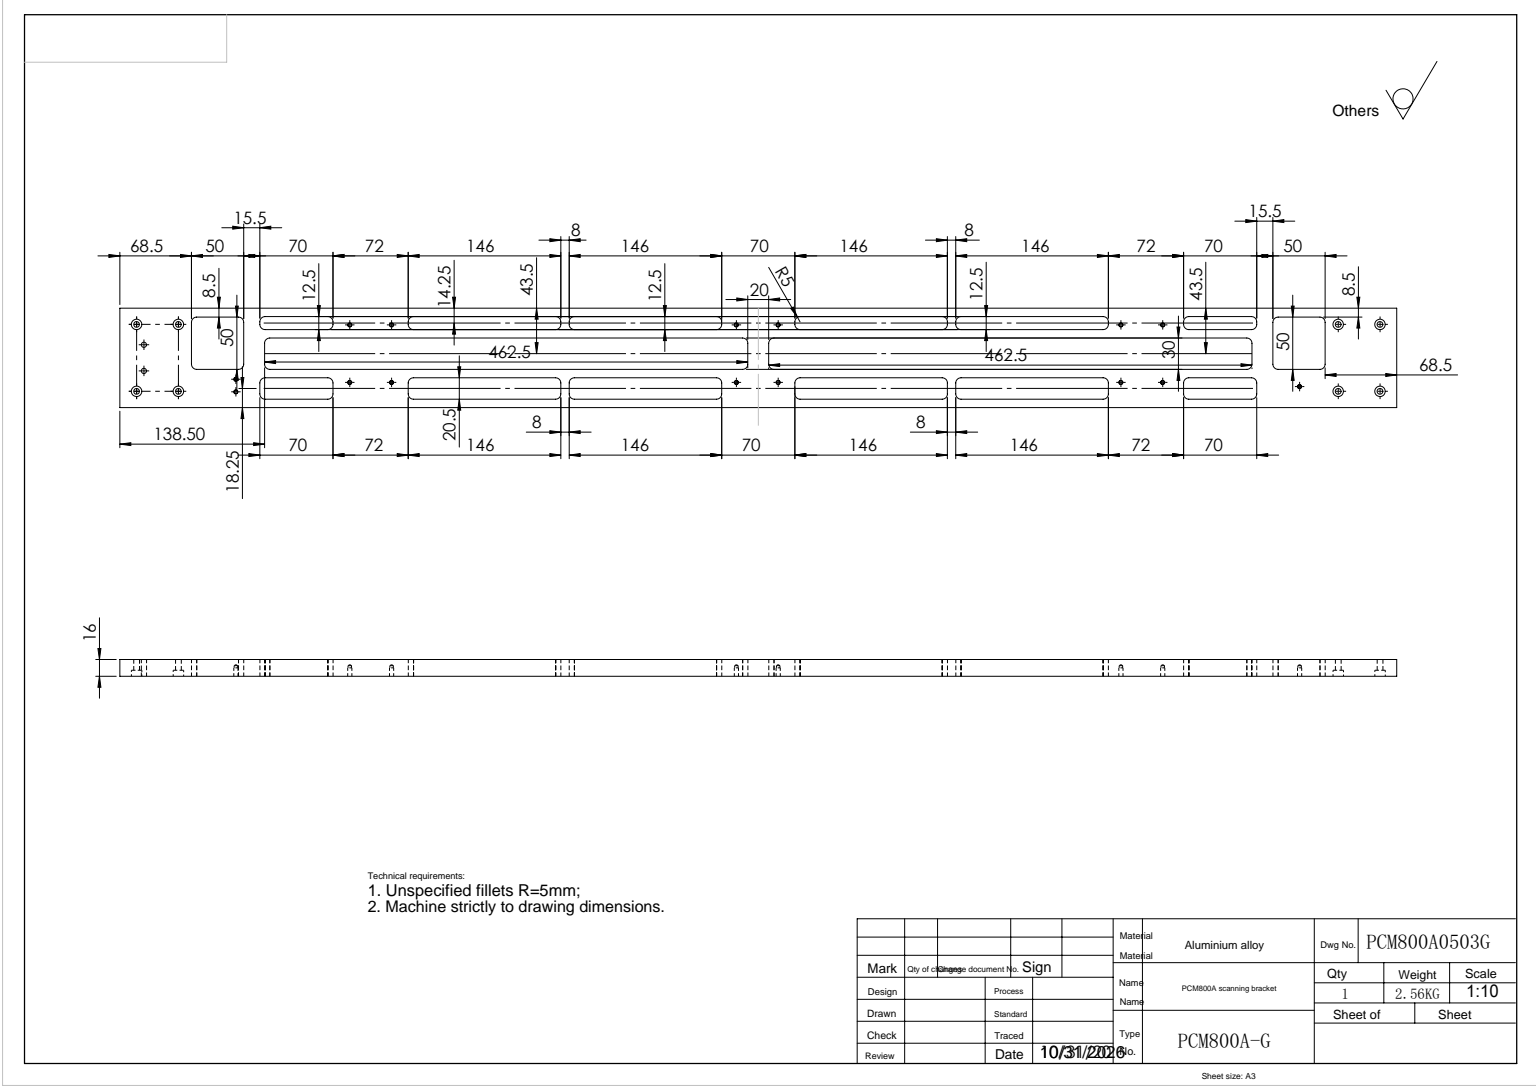
from build123d import *

# Parameters (mm, degrees)
SKETCH_1_W                           = 95
SKETCH_1_H                           = 16
EXTRUDE_1_DEPTH                      = 1222
HOLE_WIZARD_1_D                      = 5.5
HOLE_WIZARD_1_CBORE_D                = 10
HOLE_WIZARD_1_CBORE_DEPTH            = 5.7
PATTERN_LINEAR_1_COUNT               = 2
PATTERN_LINEAR_1_PITCH               = 40
PATTERN_LINEAR_1_COUNT_DIR2          = 2
PATTERN_LINEAR_1_PITCH_DIR2          = 64
HOLE_WIZARD_M5_1_D                   = 5
PATTERN_LINEAR_18_COUNT              = 2
PATTERN_LINEAR_18_PITCH              = 1150
PATTERN_LINEAR_18_COPY_1_D           = 5.5
PATTERN_LINEAR_18_COPY_1_CBORE_D     = 10
PATTERN_LINEAR_18_COPY_1_CBORE_DEPTH = 5.7
PATTERN_LINEAR_18_COPY_2_D           = 5.5
PATTERN_LINEAR_18_COPY_2_CBORE_D     = 10
PATTERN_LINEAR_18_COPY_2_CBORE_DEPTH = 5.7
PATTERN_LINEAR_18_COPY_3_D           = 5.5
PATTERN_LINEAR_18_COPY_3_CBORE_D     = 10
PATTERN_LINEAR_18_COPY_3_CBORE_DEPTH = 5.7
HOLE_WIZARD_M4_1_D                   = 3.3
HOLE_WIZARD_M4_1_DEPTH               = 10.1
HOLE_WIZARD_M4_1_CBORE_D             = 4
HOLE_WIZARD_M4_1_CBORE_DEPTH         = 8
HOLE_WIZARD_M4_1_TIP                 = 0.991420021
SKETCH_20_W                          = 30
SKETCH_20_H                          = 462.5
SKETCH_20_W_2                        = 50
SKETCH_20_H_2                        = 50
SKETCH_20_W_3                        = 20.5
SKETCH_20_H_3                        = 146
SKETCH_20_H_4                        = 70
SKETCH_20_W_4                        = 12.5
CUT_EXTRUDE_1_DEPTH                  = 158
FILLET_1_R                           = 5


with BuildPart() as part:
    # 草图1 → 拉伸1 (new body)
    with BuildSketch(Plane.XY):
        with Locations((47.5, 8)):
            Rectangle(SKETCH_1_W, SKETCH_1_H)
    extrude(amount=EXTRUDE_1_DEPTH)

    # 打孔尺寸根据内六角圆柱头螺钉的类型1 (through all)
    with Locations(Plane(origin=(15.5, 16, 16), x_dir=(0, 0, 1), z_dir=(0, 1, 0))):
        with Locations((0, 0)):
            hole_wizard_1 = CounterBoreHole(HOLE_WIZARD_1_D / 2, HOLE_WIZARD_1_CBORE_D / 2, HOLE_WIZARD_1_CBORE_DEPTH)

    # 阵列(线性)1: Hole Wizard 1 2 × 2
    with Locations(*[(j * PATTERN_LINEAR_1_PITCH_DIR2, 0, i * PATTERN_LINEAR_1_PITCH) for i in range(PATTERN_LINEAR_1_COUNT) for j in range(PATTERN_LINEAR_1_COUNT_DIR2) if (i, j) != (0, 0)]):
        add(hole_wizard_1, mode=Mode.SUBTRACT)

    # M5 螺纹孔1 (through all)
    with Locations(Plane(origin=(35, 16, 23), x_dir=(0, 0, 1), z_dir=(0, 1, 0))):
        with Locations((0, 0), (0, 25)):
            Hole(HOLE_WIZARD_M5_1_D / 2)

    # 阵列(线性)18: 打孔尺寸根据内六角圆柱头螺钉的类型1 ×2
    with Locations(*[(0, 0, i * PATTERN_LINEAR_18_PITCH) for i in range(1, PATTERN_LINEAR_18_COUNT)]):
        add(hole_wizard_1, mode=Mode.SUBTRACT)

    # 阵列(线性)18 copy 1 (through all)
    with Locations(Plane(origin=(79.5, 16, 1166), x_dir=(0, 0, 1), z_dir=(0, 1, 0))):
        with Locations((0, 0)):
            CounterBoreHole(PATTERN_LINEAR_18_COPY_1_D / 2, PATTERN_LINEAR_18_COPY_1_CBORE_D / 2, PATTERN_LINEAR_18_COPY_1_CBORE_DEPTH)

    # 阵列(线性)18 copy 2 (through all)
    with Locations(Plane(origin=(15.5, 16, 1206), x_dir=(0, 0, 1), z_dir=(0, 1, 0))):
        with Locations((0, 0)):
            CounterBoreHole(PATTERN_LINEAR_18_COPY_2_D / 2, PATTERN_LINEAR_18_COPY_2_CBORE_D / 2, PATTERN_LINEAR_18_COPY_2_CBORE_DEPTH)

    # 阵列(线性)18 copy 3 (through all)
    with Locations(Plane(origin=(79.5, 16, 1206), x_dir=(0, 0, 1), z_dir=(0, 1, 0))):
        with Locations((0, 0)):
            CounterBoreHole(PATTERN_LINEAR_18_COPY_3_D / 2, PATTERN_LINEAR_18_COPY_3_CBORE_D / 2, PATTERN_LINEAR_18_COPY_3_CBORE_DEPTH)

    # M4 螺纹孔1
    with Locations(Plane(origin=(0, 16, 0), x_dir=(-1, 0, 0), z_dir=(0, 1, 0))):
        with Locations((-79, 260), (-79, 220), (-24, 220), (-24, 260), (-79, 630), (-24, 590), (-79, 590), (-24, 630), (-79, 958), (-24, 958), (-79, 998), (-24, 998), (-20, 1129), (-27, 111), (-15, 111)):
            CounterBoreHole(HOLE_WIZARD_M4_1_D / 2, HOLE_WIZARD_M4_1_CBORE_D / 2, HOLE_WIZARD_M4_1_CBORE_DEPTH, depth=HOLE_WIZARD_M4_1_DEPTH)
            with Locations((0, 0, -(HOLE_WIZARD_M4_1_DEPTH + HOLE_WIZARD_M4_1_TIP / 2))):  # 118° drill point
                Cone(0, HOLE_WIZARD_M4_1_D / 2, HOLE_WIZARD_M4_1_TIP, mode=Mode.SUBTRACT)

    # 草图20 → 切除-拉伸1 (cut)
    with BuildSketch(Plane(origin=(0, 16, 0), x_dir=(1, 0, 0), z_dir=(0, 1, 0))):
        with Locations((51.5, -369.75)):
            Rectangle(SKETCH_20_W, SKETCH_20_H)
        with Locations((51.5, -852.25)):
            Rectangle(SKETCH_20_W, SKETCH_20_H)
        with Locations((61.5, -1128.5)):
            Rectangle(SKETCH_20_W_2, SKETCH_20_H_2)
        with Locations((61.5, -93.5)):
            Rectangle(SKETCH_20_W_2, SKETCH_20_H_2)
        with Locations((18.25, -349)):
            Rectangle(SKETCH_20_W_3, SKETCH_20_H_3)
        with Locations((18.25, -503)):
            Rectangle(SKETCH_20_W_3, SKETCH_20_H_3)
        with Locations((18.25, -169)):
            Rectangle(SKETCH_20_W_3, SKETCH_20_H_4)
        with Locations((80.75, -169)):
            Rectangle(SKETCH_20_W_4, SKETCH_20_H_4)
        with Locations((80.75, -349)):
            Rectangle(SKETCH_20_W_4, SKETCH_20_H_3)
        with Locations((80.75, -503)):
            Rectangle(SKETCH_20_W_4, SKETCH_20_H_3)
        with Locations((80.75, -1053)):
            Rectangle(SKETCH_20_W_4, SKETCH_20_H_4)
        with Locations((18.25, -1053)):
            Rectangle(SKETCH_20_W_3, SKETCH_20_H_4)
        with Locations((80.75, -873)):
            Rectangle(SKETCH_20_W_4, SKETCH_20_H_3)
        with Locations((18.25, -873)):
            Rectangle(SKETCH_20_W_3, SKETCH_20_H_3)
        with Locations((18.25, -719)):
            Rectangle(SKETCH_20_W_3, SKETCH_20_H_3)
        with Locations((80.75, -719)):
            Rectangle(SKETCH_20_W_4, SKETCH_20_H_3)
    extrude(amount=-CUT_EXTRUDE_1_DEPTH, mode=Mode.SUBTRACT)

    # 圆角1
    fillet_1_edges = [part.edges().sort_by_distance(p)[0] for p in [
        (66.5, 8, 138.5),
        (66.5, 8, 601),
        (36.5, 8, 601),
        (36.5, 8, 138.5),
        (36.5, 8, 1083.5),
        (36.5, 8, 621),
        (66.5, 8, 621),
        (66.5, 8, 1083.5),
        (36.5, 8, 1153.5),
        (36.5, 8, 1103.5),
        (86.5, 8, 1103.5),
        (86.5, 8, 1153.5),
        (36.5, 8, 118.5),
        (36.5, 8, 68.5),
        (86.5, 8, 68.5),
        (86.5, 8, 118.5),
        (8, 8, 422),
        (8, 8, 276),
        (28.5, 8, 276),
        (28.5, 8, 422),
        (28.5, 8, 430),
        (28.5, 8, 576),
        (8, 8, 576),
        (8, 8, 430),
        (8, 8, 204),
        (8, 8, 134),
        (28.5, 8, 134),
        (28.5, 8, 204),
        (74.5, 8, 204),
        (74.5, 8, 134),
        (87, 8, 134),
        (87, 8, 204),
        (74.5, 8, 422),
        (74.5, 8, 276),
        (87, 8, 276),
        (87, 8, 422),
        (87, 8, 430),
        (87, 8, 576),
        (74.5, 8, 576),
        (74.5, 8, 430),
        (74.5, 8, 1088),
        (74.5, 8, 1018),
        (87, 8, 1018),
        (87, 8, 1088),
        (8, 8, 1088),
        (8, 8, 1018),
        (28.5, 8, 1018),
        (28.5, 8, 1088),
        (74.5, 8, 946),
        (74.5, 8, 800),
        (87, 8, 800),
        (87, 8, 946),
        (8, 8, 946),
        (8, 8, 800),
        (28.5, 8, 800),
        (28.5, 8, 946),
        (28.5, 8, 792),
        (8, 8, 792),
        (8, 8, 646),
        (28.5, 8, 646),
        (74.5, 8, 792),
        (74.5, 8, 646),
        (87, 8, 646),
        (87, 8, 792),
    ]]
    fillet(fillet_1_edges, radius=FILLET_1_R)


solid = part.part
